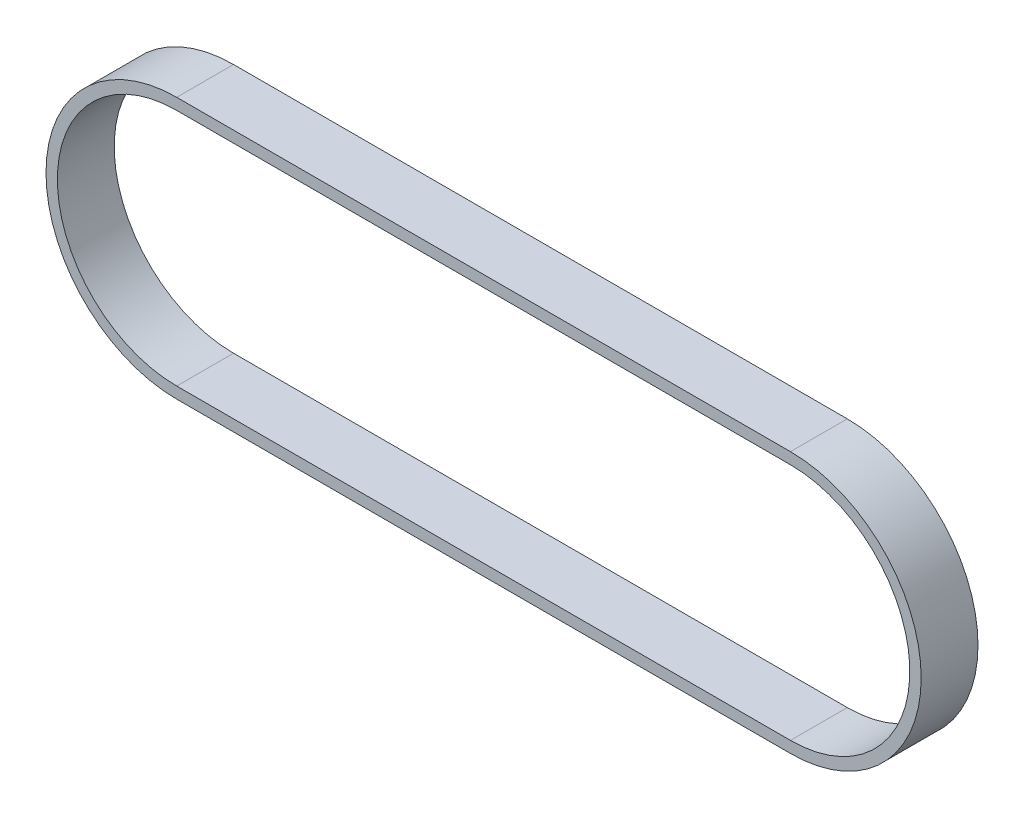
from build123d import *

# Parameters (mm, degrees)
EXTRUDE_1_DEPTH = 5


with BuildPart() as part:
    # 草图1 → 拉伸-薄壁1 (new, symmetric)
    with BuildSketch(Plane.XY):
        with BuildLine():
            Line((108, -23), (0, -23))
            ThreePointArc((0, -23), (-23, 0), (0, 23))
            Line((0, 23), (108, 23))
            ThreePointArc((108, 23), (131, 0), (108, -23))
        make_face()
        with BuildLine():
            Line((108, -21), (0, -21))
            ThreePointArc((0, -21), (-21, 0), (0, 21))
            Line((0, 21), (108, 21))
            ThreePointArc((108, 21), (129, 0), (108, -21))
        make_face(mode=Mode.SUBTRACT)
    extrude(amount=EXTRUDE_1_DEPTH, both=True)


solid = part.part
